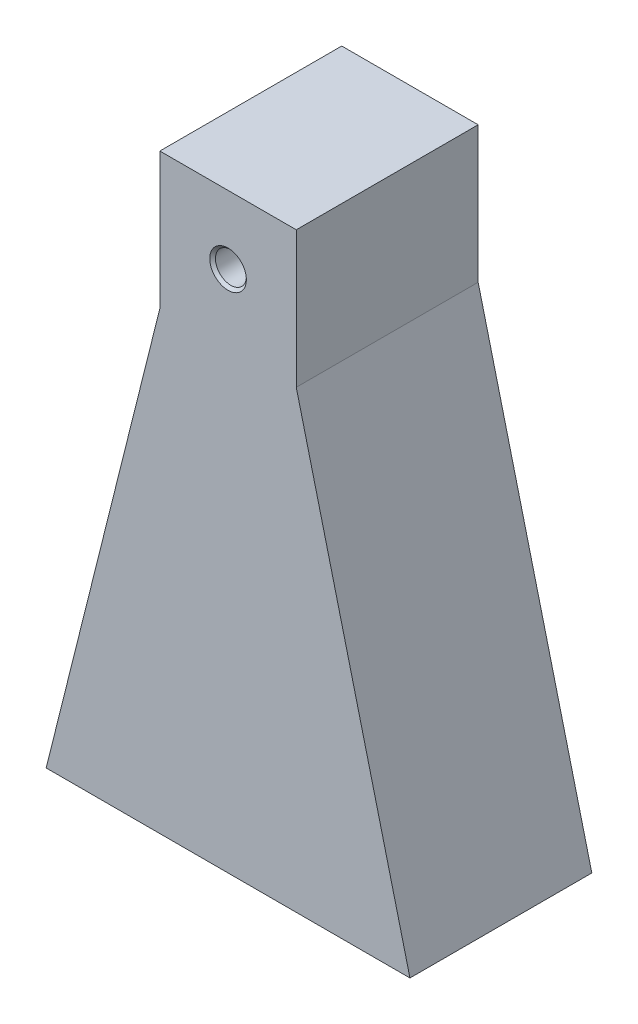
SolidWorks part; units mm, degrees
material "6061-T6 (GB)"
ref_plane "Front Plane" through (0, 0, 0) normal (0, 0, 1) x (1, 0, 0)
ref_plane "Top Plane" through (0, 0, 0) normal (0, 1, 0) x (1, 0, 0)
ref_plane "Right Plane" through (0, 0, 0) normal (1, 0, 0) x (0, 0, -1)
sketch "Sketch1" plane through (0, 0, 0) normal (0, 0, 1) x (1, 0, 0)
  line L0 (0, 0) -> (0, -72.7273) construction
  line L1 (40, -72.7273) -> (-40, -72.7273)
  line L2 (40, -72.7273) -> (15, 27.2727)
  line L3 (15, 27.2727) -> (-15, 27.2727) construction
  line L4 (-40, -72.7273) -> (-15, 27.2727)
  line L5 (40, -72.7273) -> (-15, 27.2727) construction
  line L6 (15, 27.2727) -> (-40, -72.7273) construction
  line L7 (-15, 27.2727) -> (-15, 57.2727)
  line L8 (-15, 57.2727) -> (15, 57.2727)
  line L9 (15, 57.2727) -> (15, 27.2727)
  point P0 (0, 0)
  dimension "D1" = 30
  dimension "D2" = 100
  dimension "D3" = 80
  dimension "D4" = 27.2727
  dimension "D5" = 30
extrude "Boss-Extrude1" add sketch "Sketch1" along normal blind 40
hole_wizard "M8 Tapped Hole1" positions "Sketch2" profile "Sketch3" tap size "M8" standard "GB" end condition through all
sketch "Sketch2" plane through (0, 0, 40) normal (0, 0, 1) x (1, 0, 0)
  line L0 (-15, 57.2727) -> (15, 27.2727) construction
  point P0 (0, 42.2727)
sketch "Sketch3" plane through (0, 42.2727, 40) normal (1, 0, 0) x (0, -1, 0)
  line L0 (0, 0) -> (0, 40)
  line L1 (0, 40) -> (3.4, 40)
  line L2 (3.4, 40) -> (3.4, 0.625)
  line L3 (3.4, 0.625) -> (4.025, 0)
  line L5 (4.025, 0) -> (0, 0)
  line L6 (-3.4, 0.625) -> (-4.025, 0) construction
  line L11 (0, -6.35) -> (0, 107.95) construction
  dimension "通孔螺纹孔钻头直径" = 6.8
  dimension "通孔螺纹孔钻头深度" = 40
  dimension "近端锥形沉头孔直径" = 8.05
  dimension "近端锥形沉头孔角度" = 90
cosmetic thread "Cosmetic Thread1" parameters "D2"=8
